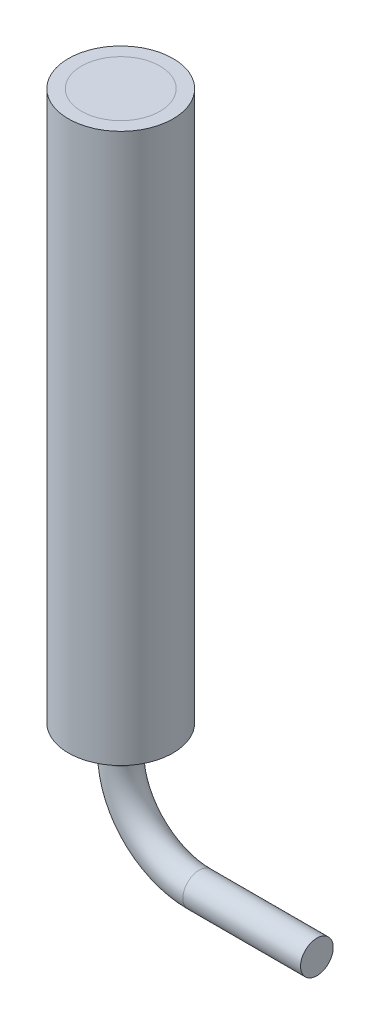
SolidWorks part; units mm, degrees
ref_plane "Front Plane" through (0, 0, 0) normal (0, 0, 1) x (1, 0, 0)
ref_plane "Top Plane" through (0, 0, 0) normal (0, 1, 0) x (1, 0, 0)
ref_plane "Right Plane" through (0, 0, 0) normal (1, 0, 0) x (0, 0, -1)
sketch "Sketch1" plane through (0, 0, 0) normal (0, 1, 0) x (1, 0, 0)
  circle A0 centre (0, 0) radius 4
  dimension "D1" = 8
extrude "Boss-Extrude1" add sketch "Sketch1" along normal blind 42
cosmetic thread "Cosmetic Thread1" parameters "D1"=33, "D2"=6.891
sketch "Sketch2" plane through (0, 0, 0) normal (0, -1, 0) x (1, 0, 0)
  circle A0 centre (0, 0) radius 1.25
  dimension "D1" = 2.5
sketch "Sketch3" plane through (0, 0, 0) normal (0, 0, 1) x (1, 0, 0)
  line L0 (0, 0) -> (0, -2)
  line L1 (6, -8) -> (15, -8)
  arc A0 (0, -2) -> (6, -8) centre (6, -2) ccw
  point P6 (0, -8)
  dimension "D3" = 6
  dimension "D1" = 8
  dimension "D2" = 15
sweep "Sweep1" add profiles "Sketch2" path "Sketch3"
sketch "Sketch4" plane through (0, 42, 0) normal (0, 1, 0) x (1, 0, 0)
  circle A0 centre (0, 0) radius 3
  dimension "D1" = 6
split line "Split Line1"
